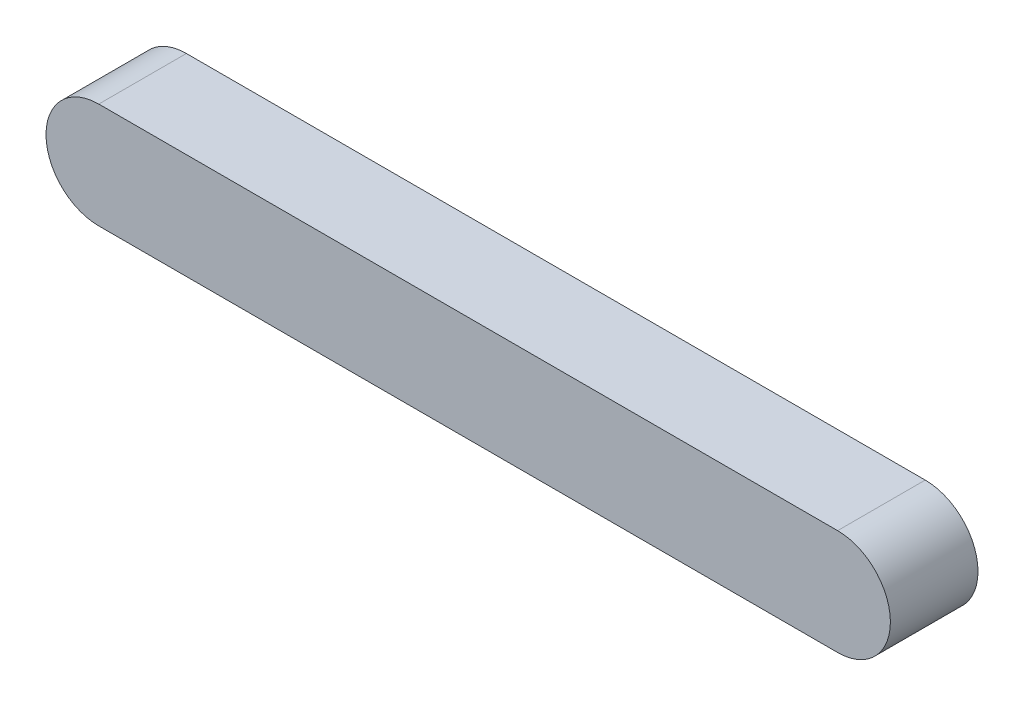
from build123d import *

# Parameters (mm, degrees)
EXTRUDE_1_DEPTH = 8.3


with BuildPart() as part:
    # 草图1 → 凸台-拉伸1 (new body)
    with BuildSketch(Plane.XY):
        with BuildLine():
            Line((0, 5), (70, 5))
            ThreePointArc((70, 5), (75, 0), (70, -5))
            Line((70, -5), (0, -5))
            ThreePointArc((0, -5), (-5, 0), (0, 5))
        make_face()
    extrude(amount=EXTRUDE_1_DEPTH)


solid = part.part
